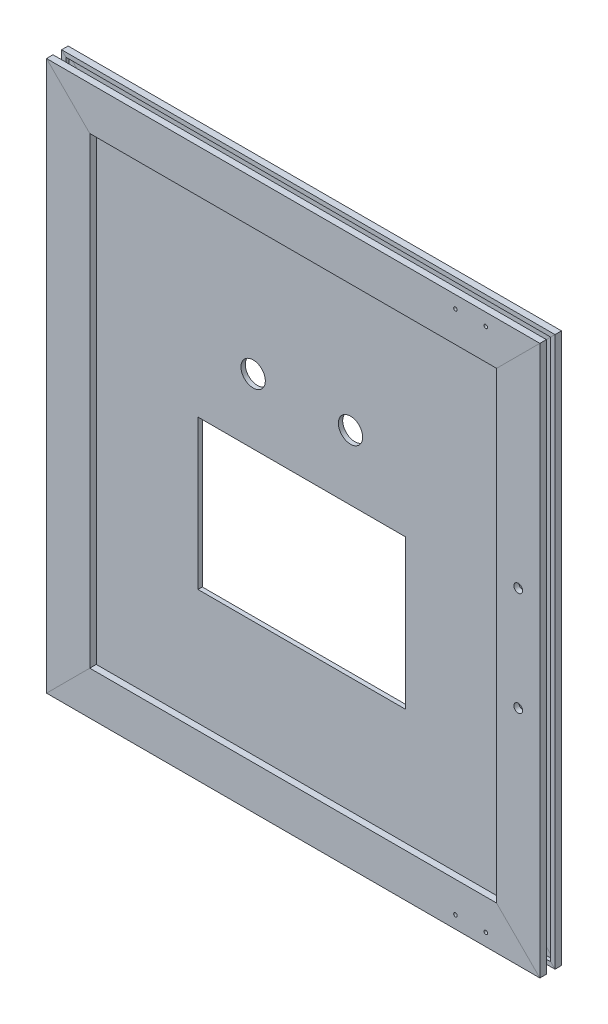
SolidWorks part; units mm, degrees
material "铝型材"
ref_plane "前视基准面" through (0, 0, 0) normal (0, 0, 1) x (1, 0, 0)
ref_plane "上视基准面" through (0, 0, 0) normal (0, 1, 0) x (1, 0, 0)
ref_plane "右视基准面" through (0, 0, 0) normal (1, 0, 0) x (0, 0, -1)
sketch "草图13" plane through (0, 0, 0) normal (0, 0, 1) x (1, 0, 0)
  line L1 (-208, -234) -> (208, -234)
  line L2 (-208, -234) -> (-208, 234)
  line L3 (-208, 234) -> (208, 234)
  line L4 (208, -234) -> (208, 234)
  line L5 (-208, -234) -> (208, 234) construction
  line L6 (-208, 234) -> (208, -234) construction
  point P0 (0, 0)
  dimension "D1" = 416
  dimension "D2" = 468
other "铝型材 2040A(1)"
ref_plane "基准面3" through (-208, 234, 0) normal (1, 0, 0) x (0, 1, 0)
sketch "草图19" plane through (-208, 234, 0) normal (1, 0, 0) x (0, 1, 0)
  line L0 (9, 4) -> (6, 4)
  line L1 (9, 4) -> (9, 7)
  line L2 (6, -4) -> (6, 4)
  line L3 (16, 7) -> (9, 7)
  line L4 (9, -4) -> (6, -4)
  line L5 (16, 4) -> (16, 7)
  line L6 (9, -7) -> (9, -4)
  line L7 (20, 4) -> (16, 4)
  line L8 (16, -7) -> (9, -7)
  line L9 (20, 10) -> (20, 4)
  line L10 (16, -7) -> (16, -4)
  line L11 (-20, 10) -> (20, 10)
  line L12 (20, -4) -> (16, -4)
  line L13 (-20, 4) -> (-20, 10)
  line L14 (20, -4) -> (20, -10)
  line L15 (-20, 4) -> (-16, 4)
  line L16 (20, -10) -> (-20, -10)
  line L17 (-16, 4) -> (-16, 7)
  line L18 (-20, -10) -> (-20, -4)
  line L19 (-16, 7) -> (-9, 7)
  line L20 (-20, -4) -> (-16, -4)
  line L21 (-9, 4) -> (-9, 7)
  line L22 (-16, -7) -> (-16, -4)
  line L23 (-9, 4) -> (-6, 4)
  line L24 (-16, -7) -> (-9, -7)
  line L25 (-6, -4) -> (-6, 4)
  line L26 (-9, -7) -> (-9, -4)
  line L27 (-9, -4) -> (-6, -4)
  circle A0 centre (0, 0) radius 3.25
  point P0 (0, 0)
sketch "草图14" plane through (0, 0, 0) normal (0, 0, 1) x (1, 0, 0)
  line L0 (214, 240) -> (217, 243) construction
  line L1 (-201.5, -227.5) -> (201.5, -227.5)
  line L2 (-201.5, -227.5) -> (-201.5, 227.5)
  line L3 (-201.5, 227.5) -> (201.5, 227.5)
  line L4 (201.5, -227.5) -> (201.5, 227.5)
  line L5 (-201.5, -227.5) -> (201.5, 227.5) construction
  line L6 (-201.5, 227.5) -> (201.5, -227.5) construction
  line L8 (188, 214) -> (-188, 214) construction
  point P0 (0, 0)
  dimension "D1" = 13.5
extrude "凸台-拉伸1" add sketch "草图14" along normal mid plane 4 separate body
hole_wizard "M4 螺纹孔2" positions "草图24" profile "草图25" tap size "M4" standard "GB"
sketch "草图24" plane through (0, 0, 10) normal (0, 0, -1) x (-1, 0, 0)
  line L0 (-178, 242.5) -> (-150, 242.5) construction
  line L7 (0, 0) -> (81.0682, 0) construction
  line L10 (-228, 254) -> (228, 254) construction
  line L11 (-228, -254) -> (-228, 254) construction
  point P0 (-178, 242.5)
  point P2 (-150, 242.5)
  point P29 (-150, -242.5)
  point P30 (-178, -242.5)
  dimension "D1" = 28
  dimension "D2" = 11.5
  dimension "D3" = 50
cosmetic thread "孔螺蚊线3" parameters "D1"=6, "D2"=4
cosmetic thread "孔螺蚊线4" parameters "D1"=6, "D2"=4
cosmetic thread "孔螺蚊线9" parameters "D1"=6, "D2"=4
cosmetic thread "孔螺蚊线10" parameters "D1"=6, "D2"=4
sketch "草图25" plane through (178, 242.5, 10) normal (1, 0, 0) x (0, -1, 0)
  line L0 (0, 0) -> (0, 11.0914)
  line L1 (0, 11.0914) -> (1.65, 10.1)
  line L2 (1.65, 10.1) -> (1.65, 0)
  line L5 (1.65, 0) -> (0, 0)
  line L10 (0, 11.0914) -> (-1.65, 10.1) construction
  line L11 (0, -6.35) -> (0, 107.95) construction
  dimension "螺纹孔钻头直径" = 3.3
  dimension "螺纹孔钻头深度" = 10.1
  dimension "导头角度" = 118
hole_wizard "打孔尺寸(%根据)开槽圆柱头螺钉的类型1" positions "草图26" profile "草图27" counterbore size "M4" standard "GB" end condition through all
sketch "草图26" plane through (0, 0, 10) normal (0, 0, 1) x (1, 0, 0)
  line L0 (0, 0) -> (50000, 0) construction
  line L1 (208, 424) -> (208, -49576) construction
  line L2 (228, 254) -> (188, 214) construction
  point P0 (208, 48)
  point P2 (208, -48)
  point P14 (208, 234)
  dimension "D1" = 96
sketch "草图27" plane through (208, 48, 10) normal (1, 0, 0) x (0, -1, 0)
  line L0 (0, 0) -> (0, 20)
  line L1 (0, 20) -> (2.25, 20)
  line L3 (2.25, 20) -> (2.25, 4.6)
  line L4 (2.25, 4.6) -> (4, 4.6)
  line L5 (4, 4.6) -> (4, 0)
  line L7 (4, 0) -> (0, 0)
  line L11 (0, -6.35) -> (0, 107.95) construction
  dimension "通孔孔直径" = 4.5
  dimension "通孔孔深度" = 20
  dimension "柱形沉头孔直径" = 8
  dimension "柱形沉头孔深度" = 4.6
hole_wizard "M6 螺纹孔1" positions "草图28" profile "草图29" tap size "M6" standard "GB"
sketch "草图28" plane through (0, 0, -10) normal (0, 0, -1) x (-1, 0, 0)
  line L0 (0, 0) -> (50000, 0) construction
  line L1 (208, 424) -> (208, -49576) construction
  line L2 (188, 214) -> (228, 254) construction
  line L3 (-228, 254) -> (228, 254) construction
  line L4 (208, -469.5) -> (208, 49530.5) construction
  point P0 (208, 194)
  point P2 (208, 157)
  point P12 (208, 234)
  point P19 (208, -194)
  point P20 (208, -157)
  dimension "D1" = 60
  dimension "D2" = 37
sketch "草图29" plane through (-208, 194, -10) normal (1, 0, 0) x (0, 1, 0)
  line L0 (0, 0) -> (0, 18.5022)
  line L1 (0, 18.5022) -> (2.5, 17)
  line L2 (2.5, 17) -> (2.5, 0)
  line L5 (2.5, 0) -> (0, 0)
  line L10 (0, 18.5022) -> (-2.5, 17) construction
  line L11 (0, -6.35) -> (0, 107.95) construction
  dimension "螺纹孔钻头直径" = 5
  dimension "螺纹孔钻头深度" = 17
  dimension "导头角度" = 118
cosmetic thread "孔螺蚊线5" parameters "D1"=15, "D2"=6
cosmetic thread "孔螺蚊线6" parameters "D1"=15, "D2"=6
cosmetic thread "孔螺蚊线7" parameters "D1"=15, "D2"=6
cosmetic thread "孔螺蚊线8" parameters "D1"=15, "D2"=6
sketch "草图30" plane through (0, 0, -10) normal (0, 0, -1) x (-1, 0, 0)
  line L0 (0, -40) -> (0, 0) construction
  line L5 (96, -109) -> (-96, -109)
  line L6 (96, -109) -> (96, 29)
  line L7 (96, 29) -> (-96, 29)
  line L8 (-96, -109) -> (-96, 29)
  line L9 (96, -109) -> (-96, 29) construction
  line L10 (96, 29) -> (-96, -109) construction
  point P0 (0, -40)
  dimension "D1" = 138
  dimension "D2" = 192
  dimension "D3" = 40
extrude "切除-拉伸1" cut sketch "草图30" against normal up to next
sketch "草图31" plane through (0, 0, -2) normal (0, 0, -1) x (-1, 0, 0)
  line L0 (-45, 89) -> (45, 89) construction
  line L1 (0, 29) -> (0, 89) construction
  line L2 (-96, 29) -> (96, 29) construction
  circle A0 centre (-45, 89) radius 11.25
  circle A1 centre (45, 89) radius 11.25
  dimension "D1" = 22.5
  dimension "D2" = 90
  dimension "D3" = 60
extrude "切除-拉伸2" cut sketch "草图31" against normal up to next (4 mm away)
